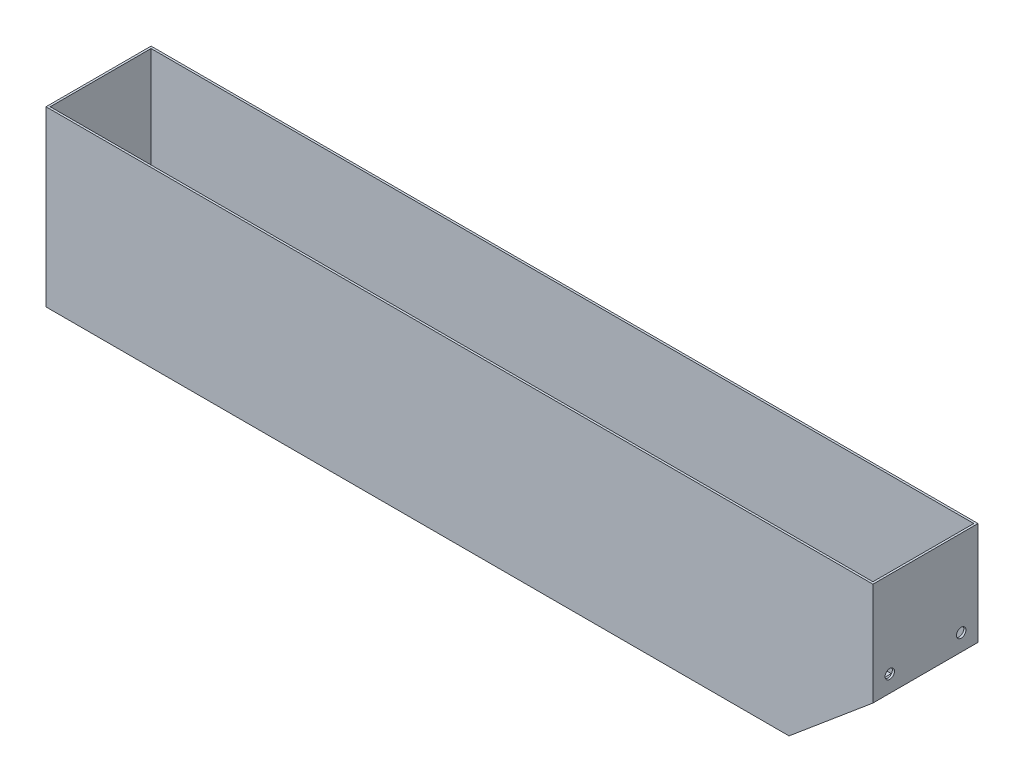
from build123d import *

# Parameters (mm, degrees)
EXTRUDE_1_DEPTH     = 100
SHELL_1_T           = -2
SKETCH_2_R          = 4.5
CUT_EXTRUDE_1_DEPTH = 10
SKETCH_3_R          = 4.5
CUT_EXTRUDE_2_DEPTH = 10


with BuildPart() as part:
    # 草图1 → 凸台-拉伸1 (new body)
    with BuildSketch(Plane.XY):
        Polygon((0, 0), (707.152509296, 0), (787, 67), (787, 165), (0, 165), align=None)
    extrude(amount=EXTRUDE_1_DEPTH)

    # 抽壳1
    shell_1_openings = [part.faces().sort_by_distance(p)[0] for p in [
        (393.5, 165, 50),
    ]]
    offset(amount=SHELL_1_T, openings=shell_1_openings, kind=Kind.INTERSECTION)

    # 草图2 → 切除-拉伸1 (cut)
    with BuildSketch(Plane.ZY):
        with Locations(Location((16, 16, 0), (0, 0, 270))):
            Circle(SKETCH_2_R)
        with Locations(Location((84, 16, 0), (0, 0, 270))):
            Circle(SKETCH_2_R)
    extrude(amount=-CUT_EXTRUDE_1_DEPTH, mode=Mode.SUBTRACT)

    # 草图3 → 切除-拉伸2 (cut)
    with BuildSketch(Plane(origin=(787, 0, 0), x_dir=(0, 0, -1), z_dir=(1, 0, 0))):
        with Locations((-84, 83)):
            Circle(SKETCH_3_R)
        with Locations((-16, 83)):
            Circle(SKETCH_3_R)
    extrude(amount=-CUT_EXTRUDE_2_DEPTH, mode=Mode.SUBTRACT)


solid = part.part
